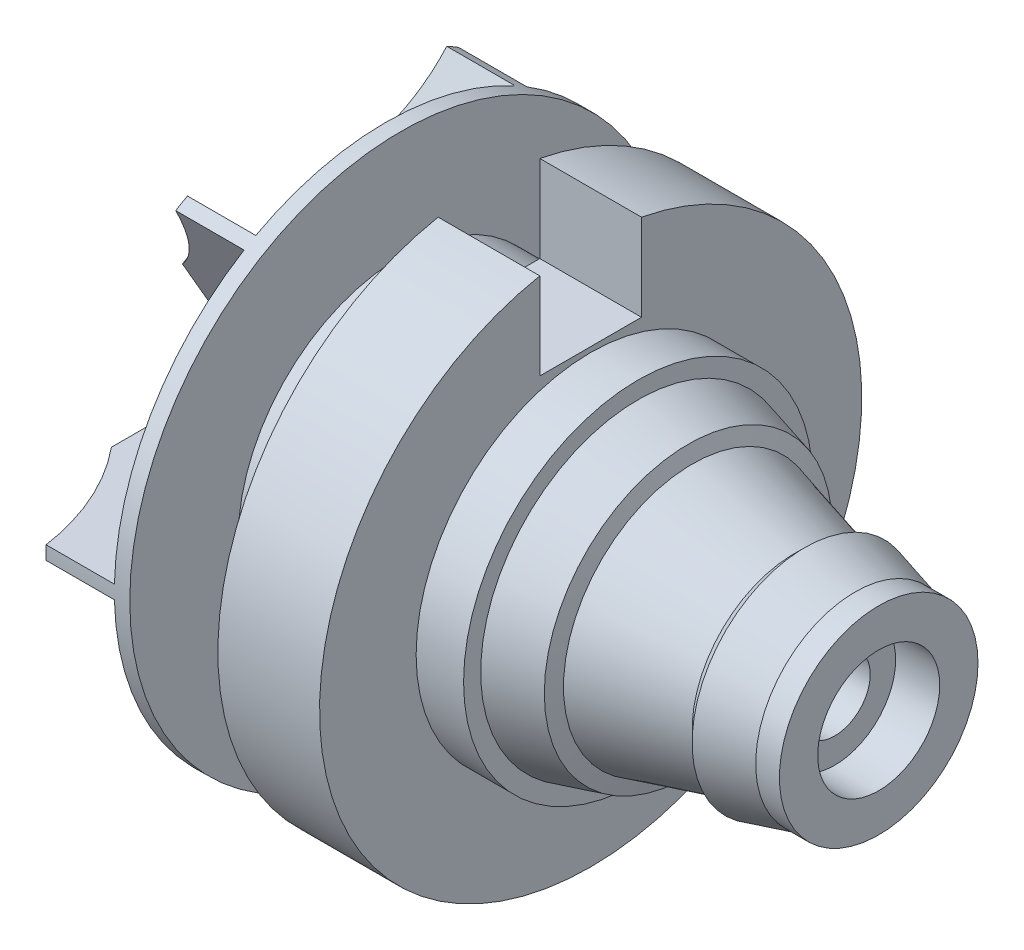
SolidWorks part; units mm, degrees
ref_plane "Front Plane" through (0, 0, 0) normal (0, 0, 1) x (1, 0, 0)
ref_plane "Top Plane" through (0, 0, 0) normal (0, 1, 0) x (1, 0, 0)
ref_plane "Right Plane" through (0, 0, 0) normal (1, 0, 0) x (0, 0, -1)
sketch "Sketch1" plane through (0, 0, 0) normal (0, 0, 1) x (1, 0, 0)
  line L0 (-6.5, 0) -> (-90.5, 0)
  line L1 (-90.5, 0) -> (-90.5, 9)
  line L2 (-72.7786, 40) -> (-70.5, 40)
  line L3 (-70.5, 40) -> (-70.5, 24)
  line L4 (-70.5, 24) -> (-57.5, 24)
  line L5 (-57.5, 24) -> (-57.5, 40)
  line L6 (-57.5, 40) -> (-42.5, 40)
  line L7 (-42.5, 40) -> (-42.5, 25.75)
  line L8 (-42.5, 25.75) -> (-35.5, 25.75)
  line L9 (-35.5, 25.75) -> (-35.5, 23.2244)
  line L10 (-35.5, 23.2244) -> (-28.1, 21.2416)
  line L11 (-3.5, 14.65) -> (0, 14.65)
  line L12 (0, 14.65) -> (0, 9)
  line L13 (0, 9) -> (-6.5, 9)
  line L14 (-6.5, 9) -> (-6.5, 0)
  line L15 (27.1454, 0) -> (-158.9634, 0) construction
  line L16 (-10.9, 16.6328) -> (-3.5, 14.65)
  line L21 (-28.1, 21.2416) -> (-27.5023, 19.0108)
  line L22 (-10.9, 16.6328) -> (-12.533, 14.9998)
  line L23 (-27.5023, 19.0108) -> (-12.533, 14.9998)
  arc A0 (-90.5, 9) -> (-72.7786, 40) centre (-117.5, 45) ccw
  point P20 (-36.0176, 21.2925)
  point P21 (-4.0176, 12.7181)
  dimension "D13" = 90
  dimension "D2" = 9
  dimension "D3" = 13
  dimension "D4" = 15
  dimension "D5" = 7
  dimension "D6" = 32
  dimension "D8" = 24
  dimension "D9" = 40
  dimension "D10" = 25.75
  dimension "D12" = 15
  dimension "D14" = 45
  dimension "D15" = 27
  dimension "D16" = 6.5
revolve "Revolve1" add sketch "Sketch1" angle 360 about L15
hole_wizard "M12x1.5 Tapped Hole1" positions "Sketch3" profile "Sketch2" tap size "M12x1.5" standard "Gb"
sketch "Sketch3" plane through (-6.5, 0, 0) normal (1, 0, 0) x (0, 0, -1)
  point P0 (0, 0)
sketch "Sketch2" plane through (-6.5, 0, 0) normal (0, 1, 0) x (0, 0, -1)
  line L0 (0, 0) -> (0, 23.1545)
  line L1 (0, 23.1545) -> (5.25, 20)
  line L2 (5.25, 20) -> (5.25, 0)
  line L5 (5.25, 0) -> (0, 0)
  line L10 (0, 23.1545) -> (-5.25, 20) construction
  line L11 (0, -6.35) -> (0, 107.95) construction
  dimension "螺纹孔钻头直径" = 10.5
  dimension "螺纹孔钻头深度" = 20
  dimension "导头角度" = 118
cosmetic thread "CosmeticThread hole thread 1" parameters "D1"=18.5, "D2"=12
sketch "Sketch4" plane through (-57.5, 0, 0) normal (-1, 0, 0) x (0, 0, 1)
  line L1 (-7.5, 39.2906) -> (-7.5, 26.5)
  line L2 (7.5, 39.2906) -> (7.5, 26.5)
  line L3 (7.5, 26.5) -> (-7.5, 26.5)
  arc A0 (7.5, 39.2906) -> (-7.5, 39.2906) centre (0, 0) ccw
  point P6 (-7.5, 40)
  point P7 (-7.5, 0)
  point P8 (7.5, 40)
  point P9 (7.5, 0)
  point P13 (38.2522, 11.6949)
extrude "Cut-Extrude1" cut sketch "Sketch4" against normal through all
sketch "Sketch5" plane through (-90.5, 0, 0) normal (-1, 0, 0) x (0, 0, 1)
  line L0 (19.1277, 35.1302) -> (3.4641, 8)
  line L1 (-39.9875, -1) -> (-8.6603, -1)
  line L2 (-39.9875, 1) -> (-8.6603, 1)
  line L3 (20.8598, 34.1302) -> (5.1962, 7)
  line L4 (20.8598, -34.1302) -> (5.1962, -7)
  line L5 (19.1277, -35.1302) -> (3.4641, -8)
  line L6 (8.6603, 1) -> (39.9875, 1)
  line L7 (-3.4641, 8) -> (-19.1277, 35.1302)
  line L8 (-5.1962, -7) -> (-20.8598, -34.1302)
  line L9 (-5.1962, 7) -> (-20.8598, 34.1302)
  line L11 (-3.4641, -8) -> (-19.1277, -35.1302)
  line L12 (8.6603, -1) -> (39.9875, -1)
  arc A0 (-39.9875, 1) -> (-39.9875, -1) centre (0, 0) ccw
  arc A1 (5.1962, -7) -> (8.6603, -1) centre (8.6603, -5) cw
  arc A2 (-8.6603, -1) -> (-5.1962, -7) centre (-8.6603, -5) cw
  arc A3 (3.4641, 8) -> (-3.4641, 8) centre (0, 10) cw
  arc A4 (-3.4641, -8) -> (3.4641, -8) centre (0, -10) cw
  arc A5 (8.6603, 1) -> (5.1962, 7) centre (8.6603, 5) cw
  arc A6 (-5.1962, 7) -> (-8.6603, 1) centre (-8.6603, 5) cw
  arc A7 (20.8598, 34.1302) -> (19.1277, 35.1302) centre (0, 0) ccw
  arc A8 (39.9875, -1) -> (39.9875, 1) centre (0, 0) ccw
  arc A9 (19.1277, -35.1302) -> (20.8598, -34.1302) centre (0, 0) ccw
  arc A10 (-20.8598, -34.1302) -> (-19.1277, -35.1302) centre (0, 0) ccw
  arc A11 (-19.1277, 35.1302) -> (-20.8598, 34.1302) centre (0, 0) ccw
  point P5 (-40, -1)
  point P6 (40, -1)
  point P7 (-40, 1)
  point P8 (40, 1)
  point P22 (0, 0)
  point P34 (0, -2)
  point P39 (-1.7321, 1)
  dimension "D2" = 4
  dimension "D1" = 3
extrude "Boss-Extrude1" add sketch "Sketch5" against normal up to surface
sketch "Sketch6" plane through (0, 0, 0) normal (0, 0, 1) x (1, 0, 0)
  line L0 (-90.5, 7.246) -> (-90.5, 34.1302) construction
  line L1 (-90.5, 1) -> (-90.5, -1) construction
  circle A0 centre (-117.5, 45) radius 35
  point P4 (-90.5, 0)
  dimension "D1" = 70
  dimension "D2" = 27
  dimension "D3" = 45
revolve "Cut-Revolve1" cut sketch "Sketch6" angle 360
